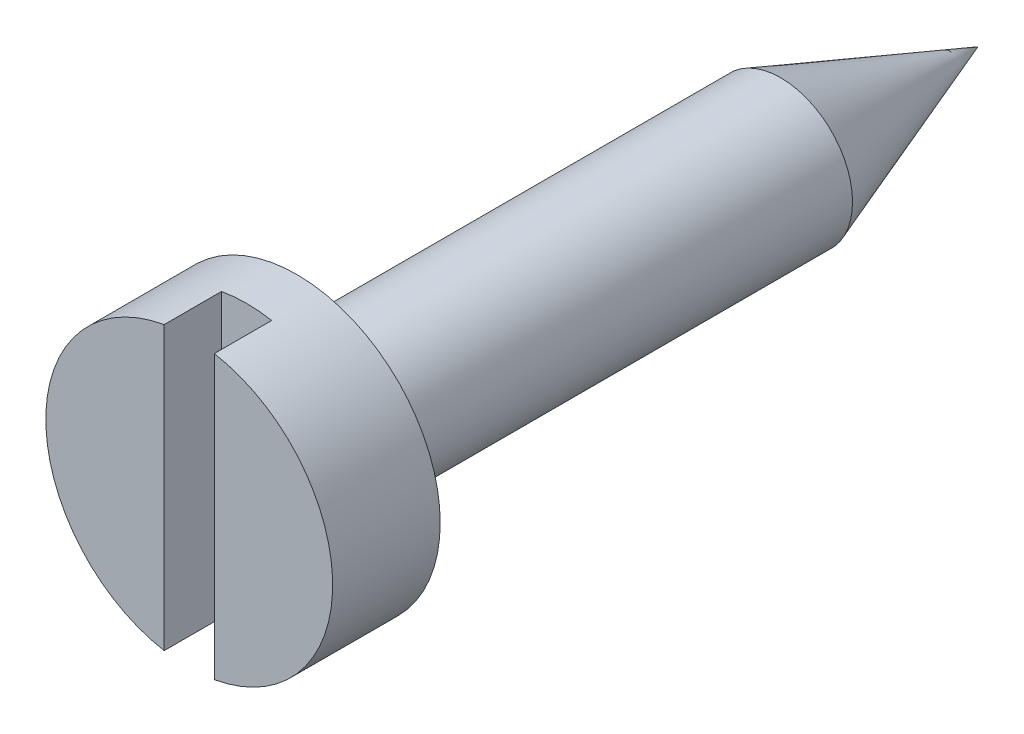
from build123d import *

# Parameters (mm, degrees)
SKETCH1_R           = 4
BOSS_EXTRUDE1_DEPTH = 3
SKETCH2_W           = 1.4
SKETCH2_H           = 9.655444372
CUT_EXTRUDE1_DEPTH  = 1.6
SKETCH3_R           = 2
BOSS_EXTRUDE2_DEPTH = 19


with BuildPart() as part:
    # Sketch1 → Boss-Extrude1 (new body)
    with BuildSketch(Plane.XY):
        Circle(SKETCH1_R)
    extrude(amount=BOSS_EXTRUDE1_DEPTH)

    # Sketch2 → Cut-Extrude1 (cut)
    with BuildSketch(Plane.XY.offset(3)):
        Rectangle(SKETCH2_W, SKETCH2_H)
    extrude(amount=-CUT_EXTRUDE1_DEPTH, mode=Mode.SUBTRACT)

    # Sketch3 → Boss-Extrude2 (add)
    with BuildSketch(Plane(origin=(0, 0, 0), x_dir=(-1, 0, 0), z_dir=(0, 0, -1))):
        Circle(SKETCH3_R)
    extrude(amount=BOSS_EXTRUDE2_DEPTH)

    # Sketch4 → Cut-Revolve5 (revolve, cut)
    with BuildSketch(Plane(origin=(0, 0, 0), x_dir=(1, 0, 0), z_dir=(0, 1, 0)), mode=Mode.PRIVATE) as cut_revolve5_sk:
        Polygon((2, 13.5), (2, 19), (0, 26.182661303), (0, 19), align=None)
    revolve(cut_revolve5_sk.sketch.rotate(Axis((0, 0, -19), (0, 0, 1)), 100.078658108), axis=Axis((0, 0, -19), (0, 0, 1)), mode=Mode.SUBTRACT)


solid = part.part
